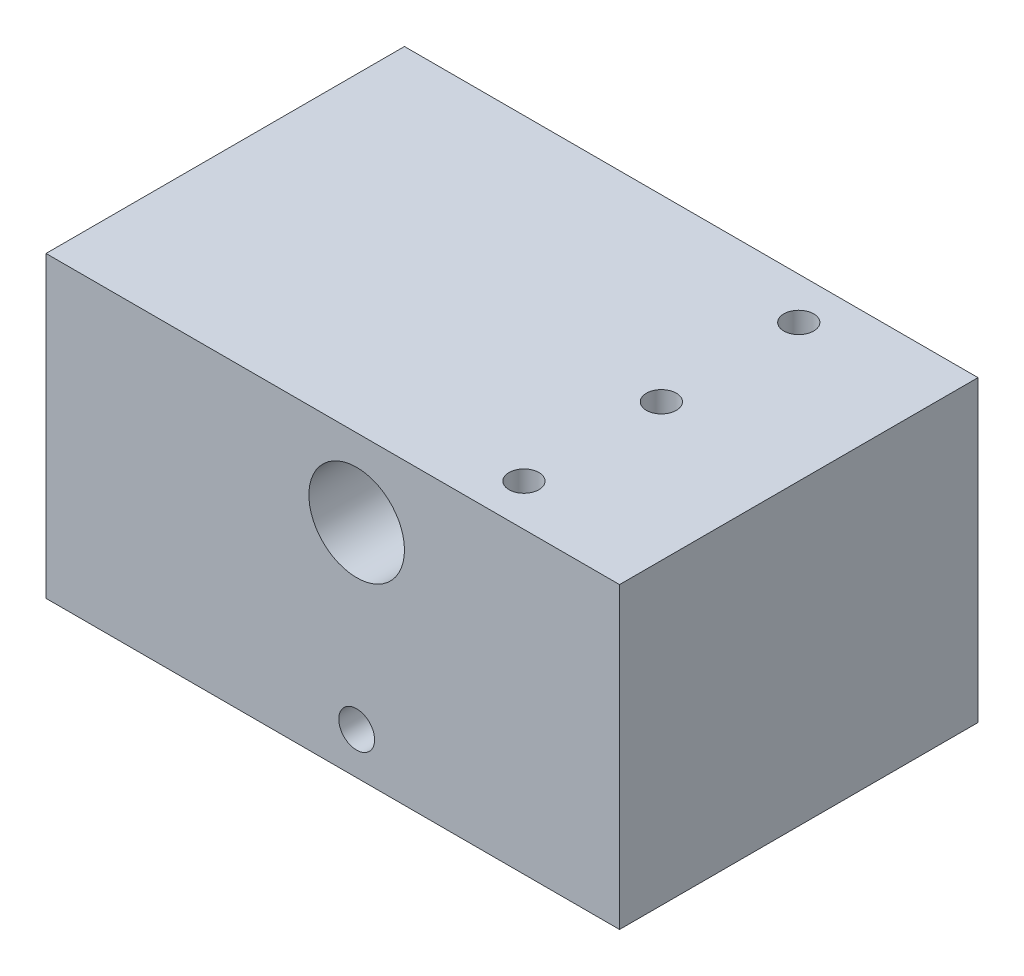
from build123d import *

# Parameters (mm, degrees)
SKETCH1_W             = 48
SKETCH1_H             = 30
BOSS_EXTRUDE1_DEPTH   = 25
CUT_EXTRUDE2_REACH    = 47.837
SKETCH3_R             = 4
SKETCH3_R_2           = 1.5
SKETCH4_R             = 1
CUT_EXTRUDE3_DEPTH    = 2
M3_TAPPED_HOLE1_D     = 2.5
M3_TAPPED_HOLE1_DEPTH = 7.5
M3_TAPPED_HOLE1_TIP   = 0.751075774


with BuildPart() as part:
    # Sketch1 → Boss-Extrude1 (new body)
    with BuildSketch(Plane(origin=(0, 0, 0), x_dir=(1, 0, 0), z_dir=(0, 1, 0))):
        Rectangle(SKETCH1_W, SKETCH1_H)
    extrude(amount=BOSS_EXTRUDE1_DEPTH)

    # Sketch3 → Cut-Extrude2 (cut, up to next)
    with BuildSketch(Plane.XY.offset(15), mode=Mode.PRIVATE) as cut_extrude2_sk1:
        with Locations((2, 18.5)):
            Circle(SKETCH3_R)
    cut_extrude2_tool1 = extrude(cut_extrude2_sk1.sketch, amount=-CUT_EXTRUDE2_REACH, mode=Mode.PRIVATE) & part.part
    # Sketch3 → Cut-Extrude2 (cut, up to next)
    with BuildSketch(Plane.XY.offset(15), mode=Mode.PRIVATE) as cut_extrude2_sk2:
        with Locations((2, 3.5)):
            Circle(SKETCH3_R_2)
    cut_extrude2_tool2 = extrude(cut_extrude2_sk2.sketch, amount=-CUT_EXTRUDE2_REACH, mode=Mode.PRIVATE) & part.part
    add(cut_extrude2_tool1.solids().sort_by_distance((2, 18.5, 15))[0], mode=Mode.SUBTRACT)
    add(cut_extrude2_tool2.solids().sort_by_distance((2, 3.5, 15))[0], mode=Mode.SUBTRACT)

    # Sketch4 → Cut-Extrude3 (cut)
    with BuildSketch(Plane(origin=(0, 25, 0), x_dir=(1, 0, 0), z_dir=(0, 1, 0))):
        with Locations(Location((12.5, 11.5, 0), (0, 0, 270))):
            Circle(SKETCH4_R)
        with Locations(Location((12.5, 0, 0), (0, 0, 270))):
            Circle(SKETCH4_R)
        with Locations(Location((12.5, -11.5, 0), (0, 0, 270))):
            Circle(SKETCH4_R)
    extrude(amount=-CUT_EXTRUDE3_DEPTH, mode=Mode.SUBTRACT)

    # M3 Tapped Hole1
    with Locations(Plane(origin=(0, 25, 0), x_dir=(1, 0, 0), z_dir=(0, 1, 0))):
        with Locations((12.5, 11.5), (12.5, 0), (12.5, -11.5)):
            Hole(M3_TAPPED_HOLE1_D / 2, depth=M3_TAPPED_HOLE1_DEPTH)
            with Locations((0, 0, -(M3_TAPPED_HOLE1_DEPTH + M3_TAPPED_HOLE1_TIP / 2))):  # 118° drill point
                Cone(0, M3_TAPPED_HOLE1_D / 2, M3_TAPPED_HOLE1_TIP, mode=Mode.SUBTRACT)


solid = part.part
